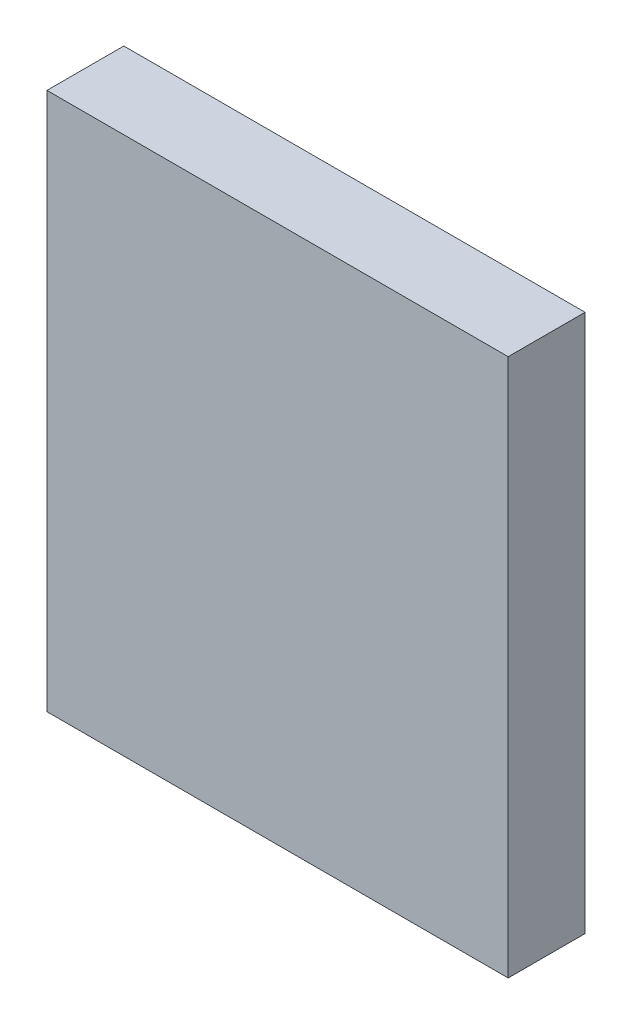
from build123d import *

# Parameters (mm, degrees)
SKETCH_1_W      = 60
SKETCH_1_H      = 70
EXTRUDE_1_DEPTH = 10


with BuildPart() as part:
    # 草图1 → 凸台-拉伸1 (new body)
    with BuildSketch(Plane.XY):
        with Locations((30, 35)):
            Rectangle(SKETCH_1_W, SKETCH_1_H)
    extrude(amount=EXTRUDE_1_DEPTH)


solid = part.part
